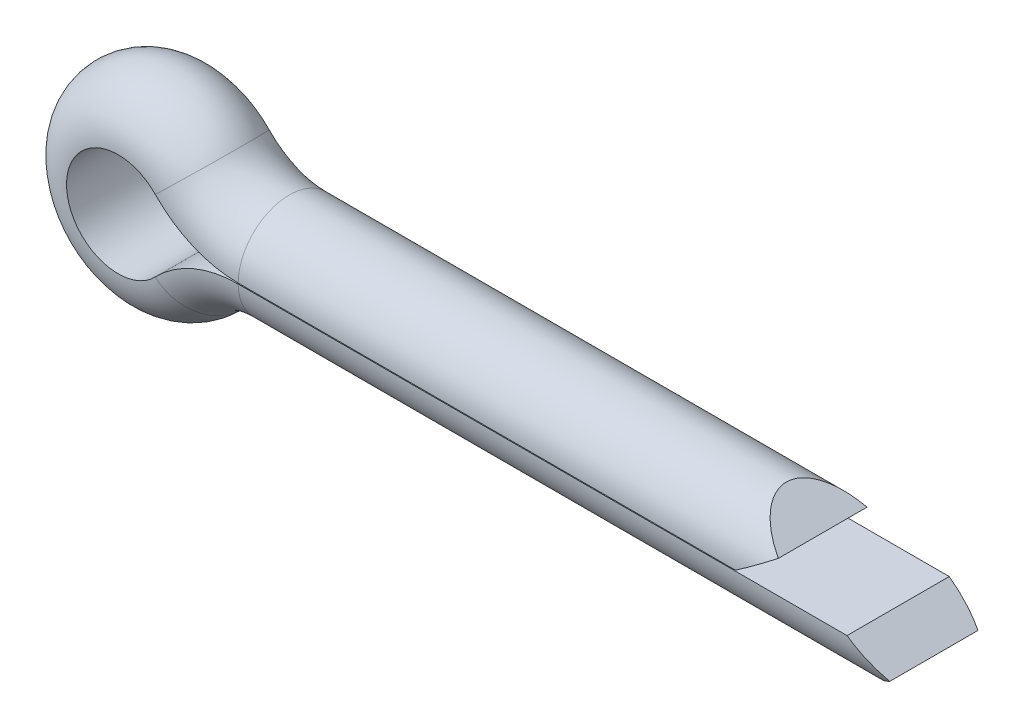
from build123d import *

# Parameters (mm, degrees)
CUT_EXTRUDE1_DEPTH      = 18.391158693
CUT_EXTRUDE1_DEPTH_BACK = 18.391158693


with BuildPart() as part:
    # Sweep2: sweep along a path in Dimension Sketch
    with BuildLine(Plane.XY) as sweep2_path:
        Line((14.7, 1.15), (2.7, 1.15))
        ThreePointArc((2.7, 1.15), (2.133929691, 1.265530578), (1.658403483, 1.593642961))
        ThreePointArc((1.658403483, 1.593642961), (-2.3, 0), (1.658403483, -1.593642961))
        ThreePointArc((1.658403483, -1.593642961), (2.133929691, -1.265530578), (2.7, -1.15))
        Line((2.7, -1.15), (17.2, -1.15))
    # Sketch2 → Sweep2 (sweep)
    with BuildSketch(Plane(origin=(14.7, 1.15, 0), x_dir=(0, 0, 1), z_dir=(-1, 0, 0))):
        with BuildLine():
            Line((-1.149956521, -1.14), (1.149956521, -1.14))
            ThreePointArc((1.149956521, -1.14), (0, 0), (-1.149956521, -1.14))
        make_face()
    sweep(path=sweep2_path.line)

    # Sketch3 → Cut-Extrude1 (cut, two sides: drawn at the far end of the back side and taken through both)
    with BuildSketch(Plane.XY.offset(-CUT_EXTRUDE1_DEPTH_BACK)):
        Polygon((14.7, 0.57), (13.882315934, 1.15), (17.21, 1.15), (17.21, -1.15), (16.375313858, -1.15), (17.2, -0.58), (16.382315934, 0), (13.875313858, 0), align=None)
    extrude(amount=CUT_EXTRUDE1_DEPTH + CUT_EXTRUDE1_DEPTH_BACK, mode=Mode.SUBTRACT)


solid = part.part
